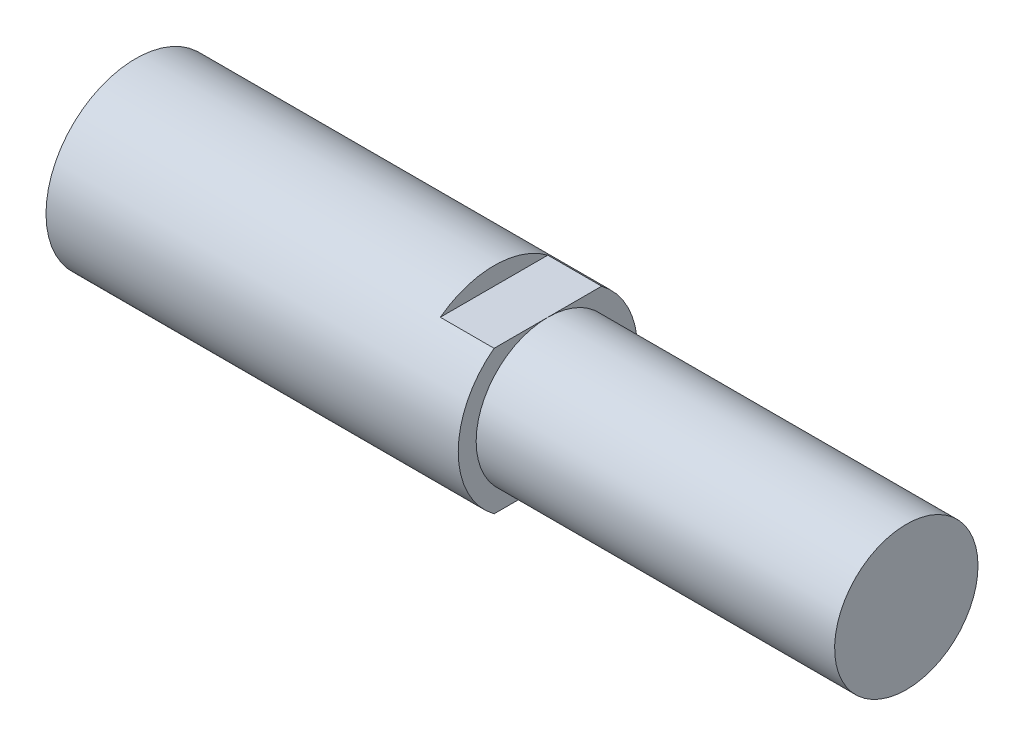
from build123d import *

# Parameters (mm, degrees)
SKETCH_1_R           = 4
EXTRUDE_1_DEPTH      = 20
SKETCH_2_R           = 5
EXTRUDE_2_DEPTH      = 3
SKETCH_3_OUTSIDE_W   = 17.4
SKETCH_3_OUTSIDE_H   = 17.4
SKETCH_3_OUTSIDE_W_2 = 14.173876264
SKETCH_3_OUTSIDE_H_2 = 8
CUT_EXTRUDE_1_DEPTH  = 25.062418831
SKETCH_4_R           = 5
EXTRUDE_3_DEPTH      = 20


with BuildPart() as part:
    # 草图1 → 凸台-拉伸1 (new body)
    with BuildSketch(Plane(origin=(0, 0, 0), x_dir=(0, 0, -1), z_dir=(1, 0, 0))):
        Circle(SKETCH_1_R)
    extrude(amount=EXTRUDE_1_DEPTH)

    # 草图2 → 凸台-拉伸2 (add)
    with BuildSketch(Plane.ZY):
        Circle(SKETCH_2_R)
    extrude(amount=EXTRUDE_2_DEPTH)

    # 草图3 outside → 切除-拉伸1 (cut, through all)
    with BuildSketch(Plane.ZY.offset(3)):
        Rectangle(SKETCH_3_OUTSIDE_W, SKETCH_3_OUTSIDE_H)
        Rectangle(SKETCH_3_OUTSIDE_W_2, SKETCH_3_OUTSIDE_H_2, mode=Mode.SUBTRACT)
    extrude(amount=-CUT_EXTRUDE_1_DEPTH, mode=Mode.SUBTRACT)

    # 草图4 → 凸台-拉伸3 (add)
    with BuildSketch(Plane.ZY.offset(3)):
        with Locations(Location((0, 0, 0), (0, 0, 126.869897646))):
            Circle(SKETCH_4_R)
    extrude(amount=EXTRUDE_3_DEPTH)


solid = part.part
